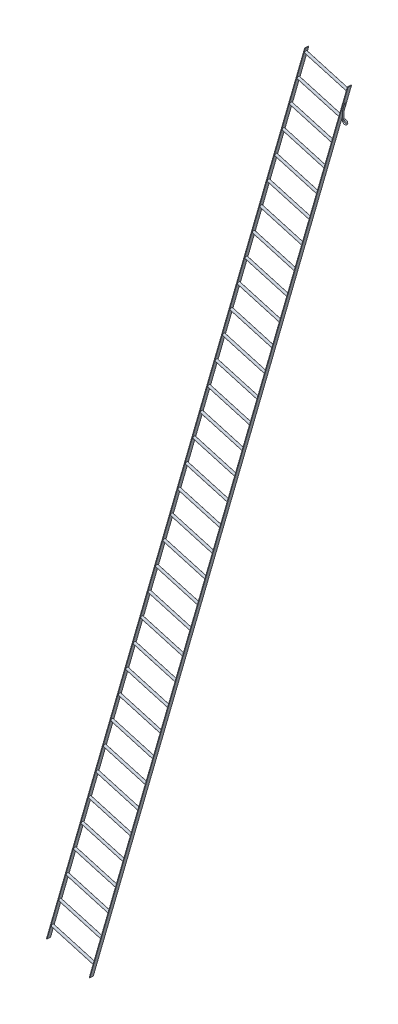
SolidWorks part; units mm, degrees
material "Q235B"
ref_plane "Front Plane" through (0, 0, 0) normal (0, 0, 1) x (1, 0, 0)
ref_plane "Top Plane" through (0, 0, 0) normal (0, 1, 0) x (1, 0, 0)
ref_plane "Right Plane" through (0, 0, 0) normal (1, 0, 0) x (0, 0, -1)
sketch "feature 17 (ProfileFeature) (+16 more in 12 files) Sketch1" plane through (0, 0, 0) normal (0, 0, 1) x (1, 0, 0)
  line L0 (-20, 0) -> (-20, 100.1568)
  line L1 (-19.7676, 101.8106) -> (2.3661, 179)
  line L2 (0, 20) -> (-13.95, 20)
  arc A0 (-20, 0) -> (0, 20) centre (0, 0) ccw
  arc A1 (-20, 100.1568) -> (-19.7676, 101.8106) centre (-14, 100.1568) cw
  point P9 (-20, 101)
  dimension "D1" = 40
  dimension "D6" = 6
  dimension "D2" = 101
  dimension "D3" = 164
  dimension "D4" = 78
  dimension "D5" = 6.05
sweep "Sweep2" add path "feature 17 (ProfileFeature) (+16 more in 12 files) Sketch1" circular profile diameter 12 parameters "D3"=12
chamfer "Chamfer1" distance 0.5 angle 45 1 edges at (-3.4014, 180.6538, 0)
sketch "0:feat:20/0 feature 20/0 (ProfileFeature) (+11 more in 7 files) Sketch2" plane through (0, 0, 0) normal (0, 0, 1) x (1, 0, 0)
  line L0 (56.1154, 366.446) -> (-424.5154, 504.2647) construction
  line L3 (-2816.2806, -9629.0218) -> (50.3479, 368.0999)
  line L4 (-3.5392, 180.1732) -> (-25.5351, 103.4644) construction
  line L5 (-424.5154, 504.2647) -> (-3291.1439, -9492.8569)
  line L6 (-3249.7983, -9348.6677) -> (-2774.935, -9484.8325)
  line L7 (-3167.1071, -9060.2892) -> (-2692.2438, -9196.454)
  line L8 (2.3661, 179) -> (56.1154, 366.446)
  line L9 (7.6531, 177.484) -> (-2.9208, 180.516) construction
  dimension "D1" = 10400
  dimension "D2" = 494
  dimension "D3" = 150
  dimension "D4" = 300
  dimension "D5" = 195
ref_plane "Plane2" through (0, 0, -20) normal (0, 0, 1) x (1, 0, 0)
sketch "Sketch7" plane through (0, 0, -20) normal (0, 0, 1) x (1, 0, 0)
  line L0 (-3167.1071, -9060.2892) -> (-2692.2438, -9196.454) construction
  line L1 (-3249.7983, -9348.6677) -> (-2774.935, -9484.8325) construction
  line L2 (-424.5154, 504.2647) -> (-3291.1439, -9492.8569) construction
  line L3 (-2816.2806, -9629.0218) -> (50.3479, 368.0999) construction
  line L4 (-3167.1071, -9060.2892) -> (-2692.2438, -9196.454)
  line L5 (-3249.7983, -9348.6677) -> (-2774.935, -9484.8325)
  line L6 (-424.5154, 504.2647) -> (-3291.1439, -9492.8569)
  line L7 (-2816.2806, -9629.0218) -> (50.3479, 368.0999)
other "Gb／t 704—1988Hot-rolled Flat Steel 40×6(1)"
ref_plane "Plane3" through (-2816.2806, -9629.0218, -20) normal (-0.2756, -0.9613, 0) x (0, 0, 1)
sketch "Sketch1" plane through (-2816.2806, -9629.0218, -20) normal (-0.2756, -0.9613, 0) x (0, 0, 1)
  line L0 (0, 0) -> (0, 6)
  line L1 (40, 0) -> (40, 6)
  line L3 (0, 6) -> (40, 6)
  line L4 (20, 6) -> (20, 0) construction
  line L5 (40, 0) -> (0, 0)
  point P1 (0, 0)
  point P10 (20, 0)
  point P16 (20, 6)
  point P18 (40, 6)
  dimension "D3" = 40
  dimension "D1" = 6
other "Gb／t 6728—2002Round Tube 26.8 X 3(2)"
ref_plane "Plane5" through (-3249.7983, -9348.6677, 0) normal (0.9613, -0.2756, 0) x (0.2756, 0.9613, 0)
sketch "Sketch13" plane through (-3249.7983, -9348.6677, 0) normal (0.9613, -0.2756, 0) x (0.2756, 0.9613, 0)
  circle A0 centre (0, 0) radius 10.4
  circle A1 centre (0, 0) radius 13.4
  point P3 (0, 0)
  dimension "Out_dia" = 26.8
  dimension "D1" = 3
  dimension "D2" = 20.8
other "Trim/Extend1"
pattern_linear "Pattern (Linear)1" count 34 spacing 300 along (0.2756, 0.9613, 0) of bodies 113
